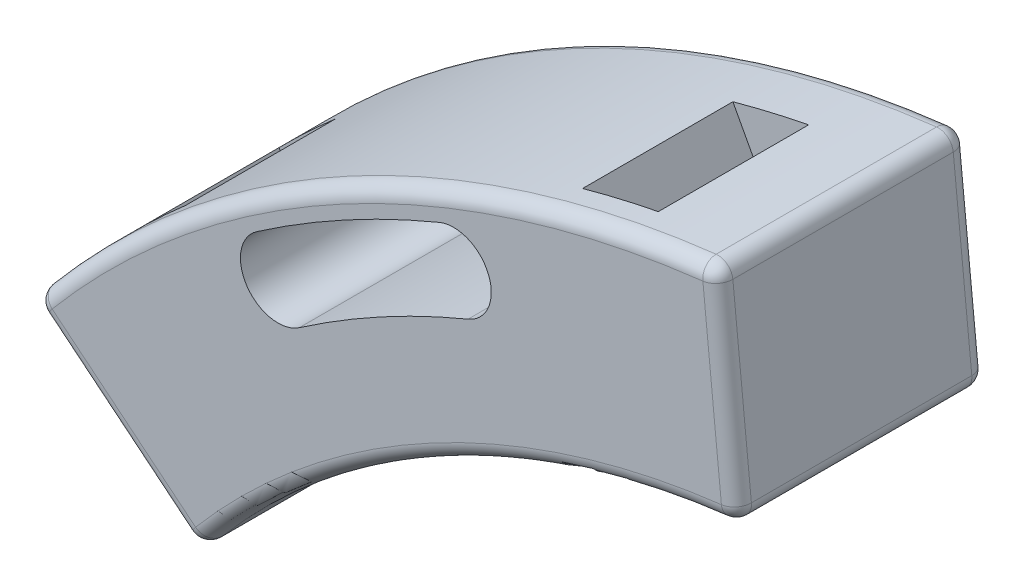
from build123d import *

# Parameters (mm, degrees)
BOSS_EXTRUDE1_DEPTH     = 50
SKETCH2_W               = 15
SKETCH2_H               = 30
CUT_EXTRUDE1_DEPTH      = 20
CUT_EXTRUDE2_DEPTH      = 594.131240453
CUT_EXTRUDE2_DEPTH_BACK = 594.131240453
FILLET1_R               = 3


with BuildPart() as part:
    # Sketch1 → Boss-Extrude1 (new body)
    with BuildSketch(Plane.XY):
        with BuildLine():
            Line((-307.585956352, 341.88779966), (-311.885113994, 384.650908092))
            ThreePointArc((-311.885113994, 384.650908092), (-387.611395489, 361.512211901), (-448.718561356, 311.155650759))
            Line((-448.718561356, 311.155650759), (-415.440513877, 283.957530324))
            ThreePointArc((-415.440513877, 283.957530324), (-367.274758623, 323.649467677), (-307.585956352, 341.88779966))
        make_face()
    extrude(amount=BOSS_EXTRUDE1_DEPTH)

    # Sketch2 → Cut-Extrude1 (cut)
    with BuildSketch(Plane(origin=(-237.484086125, 442.147798063, 0), x_dir=(0.880965905900498, 0.47317974665122253, 0), z_dir=(-0.47317974665122253, 0.880965905900498, 0))):
        with Locations((-222.912167325, -28)):
            Rectangle(SKETCH2_W, SKETCH2_H)
        with Locations((-117.912167325, -28)):
            Rectangle(SKETCH2_W, SKETCH2_H)
    extrude(amount=-CUT_EXTRUDE1_DEPTH, mode=Mode.SUBTRACT)

    # Sketch3 → Cut-Extrude2 (cut, two sides: drawn at the far end of the back side and taken through both)
    with BuildSketch(Plane(origin=(0, 0, 0), x_dir=(-1, 0, 0), z_dir=(0, 0, -1)).offset(-CUT_EXTRUDE2_DEPTH_BACK)):
        with BuildLine():
            ThreePointArc((403.644999576, 345.361735137), (385.937282785, 356.235559249), (367.185078684, 365.188666312))
            ThreePointArc((367.185078684, 365.188666312), (357.385414117, 361.130763607), (361.443316822, 351.33109904))
            ThreePointArc((361.443316822, 351.33109904), (378.77130289, 343.057974791), (395.134129798, 333.010010739))
            ThreePointArc((395.134129798, 333.010010739), (405.565426886, 334.930438049), (403.644999576, 345.361735137))
        make_face()
    extrude(amount=CUT_EXTRUDE2_DEPTH + CUT_EXTRUDE2_DEPTH_BACK, mode=Mode.SUBTRACT)

    # Fillet1
    fillet1_edges = [part.edges().sort_by_distance(p)[0] for p in [
        (-387.611395489, 361.512211901, 50),
        (-432.079537616, 297.556590541, 50),
        (-367.274758623, 323.649467677, 50),
        (-432.079537616, 297.556590541, 0),
        (-387.611395489, 361.512211901, 0),
        (-309.735535173, 363.269353876, 0),
        (-367.274758623, 323.649467677, 0),
        (-415.440513877, 283.957530324, 25),
        (-448.718561356, 311.155650759, 25),
        (-311.885113994, 384.650908092, 25),
        (-307.585956352, 341.88779966, 25),
        (-309.735535173, 363.269353876, 50),
    ]]
    fillet(fillet1_edges, radius=FILLET1_R)


solid = part.part
